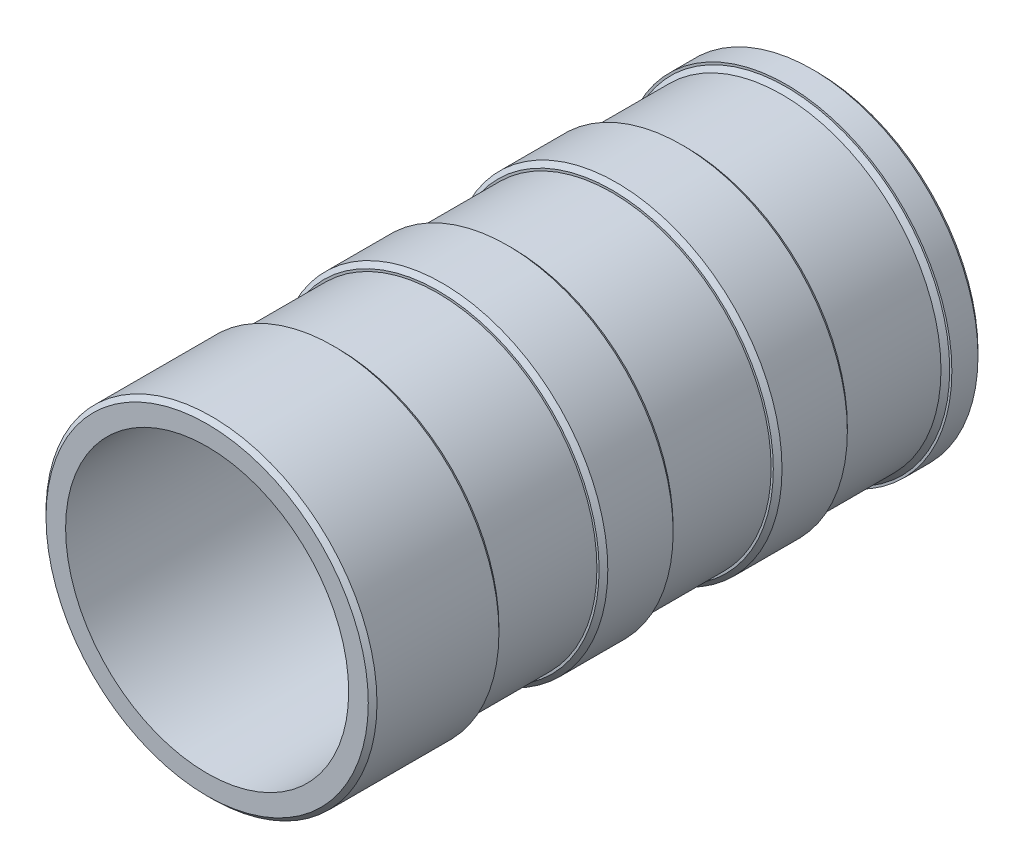
from build123d import *

# Parameters (mm, degrees)
SKETCH_1_R             = 38
SKETCH_1_R_2           = 32.5
EXTRUDE_1_DEPTH        = 140
CHAMFER_1_SIZE         = 1
CUT_EXTRUDE_START      = -23
SKETCH_2_R             = 38
SKETCH_2_R_2           = 36.5
CUT_EXTRUDE_1_DEPTH    = 23
PATTERN_LINEAR_1_COUNT = 3
PATTERN_LINEAR_1_PITCH = 40
CHAMFER_2_SIZE         = 1


with BuildPart() as part:
    # 草图1 → 凸台-拉伸1 (new body)
    with BuildSketch(Plane.XY):
        Circle(SKETCH_1_R)
        Circle(SKETCH_1_R_2, mode=Mode.SUBTRACT)
    extrude(amount=EXTRUDE_1_DEPTH)

    # 倒角1
    chamfer_1_edges = [part.edges().sort_by_distance(p)[0] for p in [
        (-38, 0, 140),
    ]]
    chamfer(chamfer_1_edges, length=CHAMFER_1_SIZE)

    # 草图2 → 切除-拉伸1 (cut)
    with BuildSketch(Plane.XY.offset(110).offset(CUT_EXTRUDE_START)):
        Circle(SKETCH_2_R)
        Circle(SKETCH_2_R_2, mode=Mode.SUBTRACT)
    cut_extrude_1 = extrude(amount=CUT_EXTRUDE_1_DEPTH, mode=Mode.SUBTRACT)

    # 阵列(线性)1: 切除-拉伸1 ×3
    with Locations(*[(0, 0, -i * PATTERN_LINEAR_1_PITCH) for i in range(1, PATTERN_LINEAR_1_COUNT)]):
        add(cut_extrude_1, mode=Mode.SUBTRACT)

    # 倒角2
    chamfer_2_edges = [part.edges().sort_by_distance(p)[0] for p in [
        (-38, 0, 87),
        (-38, 0, 110),
        (-38, 0, 0),
        (-38, 0, 47),
        (-38, 0, 70),
        (-36.5, 0, 7),
        (-38, 0, 30),
    ]]
    chamfer(chamfer_2_edges, length=CHAMFER_2_SIZE)


solid = part.part
